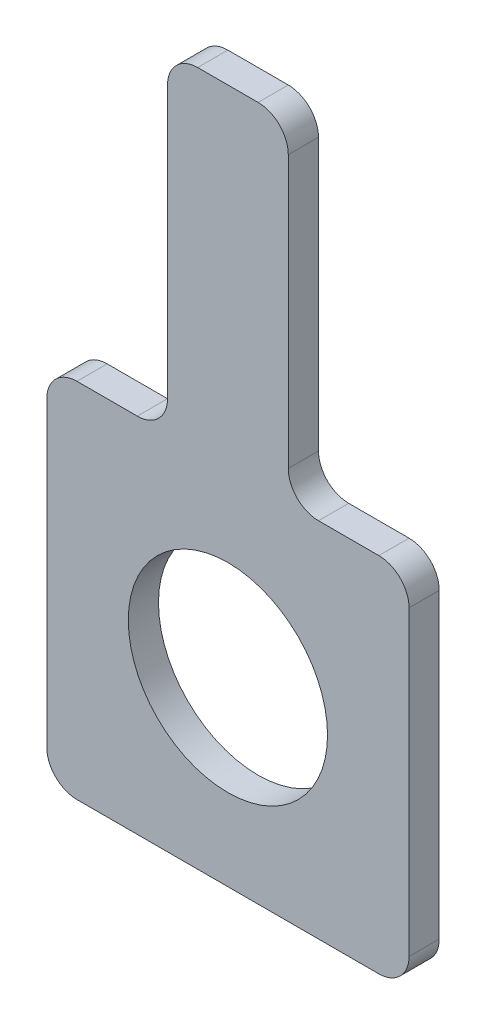
from build123d import *

# Parameters (mm, degrees)
BOSS_EXTRUDE1_DEPTH  = 1
M6_CLEARANCE_HOLE1_D = 6.6
FILLET1_R            = 1


with BuildPart() as part:
    # Sketch1 → Boss-Extrude1 (new body)
    with BuildSketch(Plane.XY):
        Polygon((2, 6), (6, 6), (6, -6), (-6, -6), (-6, 6), (-2, 6), (-2, 17), (2, 17), align=None)
    extrude(amount=BOSS_EXTRUDE1_DEPTH)

    # M6 Clearance Hole1 (through all)
    with Locations(Plane.XY.offset(1)):
        with Locations((0, 0)):
            Hole(M6_CLEARANCE_HOLE1_D / 2)

    # Fillet1
    fillet1_edges = [part.edges().sort_by_distance(p)[0] for p in [
        (6, -6, 0.5),
        (-6, -6, 0.5),
        (-6, 6, 0.5),
        (-2, 6, 0.5),
        (-2, 17, 0.5),
        (2, 17, 0.5),
        (2, 6, 0.5),
        (6, 6, 0.5),
    ]]
    fillet(fillet1_edges, radius=FILLET1_R)


solid = part.part
